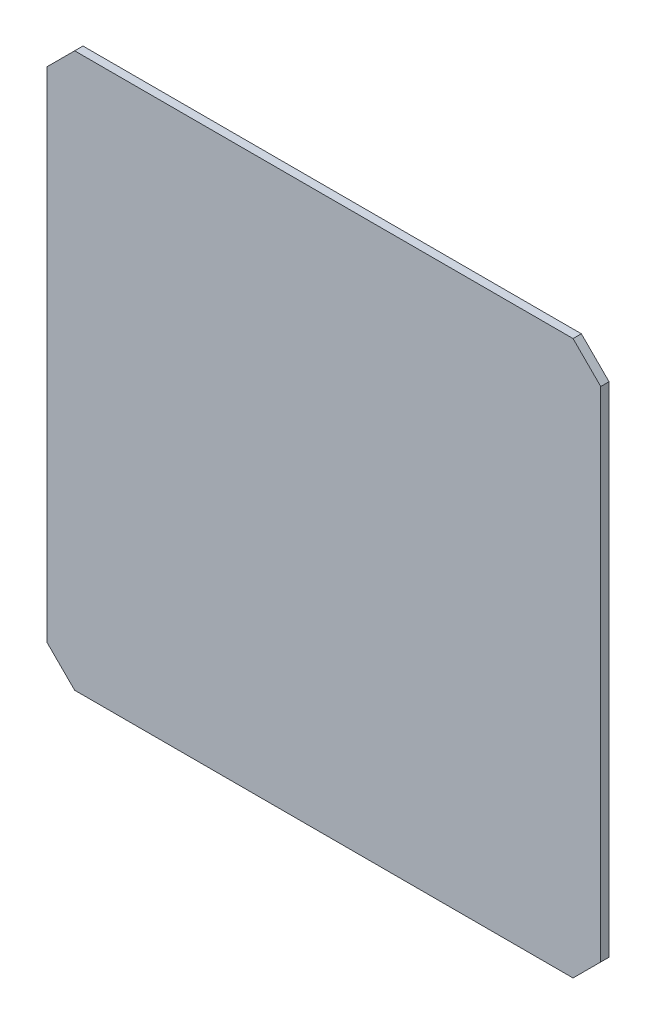
SolidWorks part; units mm, degrees
material "Q235-A"
ref_plane "前视基准面" through (0, 0, 0) normal (0, 0, 1) x (1, 0, 0)
ref_plane "上视基准面" through (0, 0, 0) normal (0, 1, 0) x (1, 0, 0)
ref_plane "右视基准面" through (0, 0, 0) normal (1, 0, 0) x (0, 0, -1)
sketch "草图1" plane through (0, 0, 0) normal (0, 0, 1) x (1, 0, 0)
  line L1 (-100, 100) -> (100, 100)
  line L2 (-100, 100) -> (-100, -100)
  line L3 (-100, -100) -> (100, -100)
  line L4 (100, 100) -> (100, -100)
  line L5 (-100, 100) -> (100, -100) construction
  line L6 (-100, -100) -> (100, 100) construction
  point P0 (0, 0)
  dimension "D1" = 200
  dimension "D2" = 200
extrude "凸台-拉伸1" add sketch "草图1" along normal blind 3
chamfer "倒角1" distance 10 angle 45 4 edges at (-100, 100, 1.5) (-100, -100, 1.5) (100, -100, 1.5) (100, 100, 1.5)
